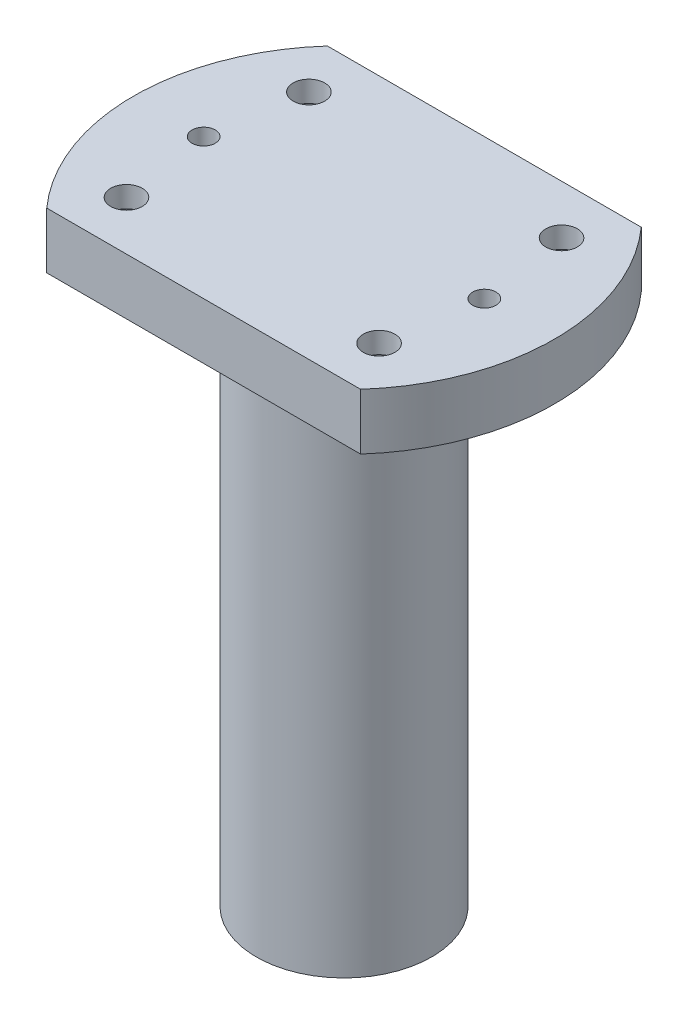
from build123d import *

# Parameters (mm, degrees)
M4_TAPPED_HOLE1_D                       = 3.3
M4_TAPPED_HOLE1_DEPTH                   = 11.5
M4_TAPPED_HOLE1_TIP                     = 0.991420021
CUT_EXTRUDE2_REACH                      = 97
CBORE_FOR_M4_HEX_HEAD_BOLT1_D           = 3
CBORE_FOR_M4_HEX_HEAD_BOLT1_CBORE_D     = 8
CBORE_FOR_M4_HEX_HEAD_BOLT1_CBORE_DEPTH = 3
M4_TAPPED_HOLE4_D                       = 3.3
M4_TAPPED_HOLE4_DEPTH                   = 10.1
M4_TAPPED_HOLE4_TIP                     = 0.991420021
CBORE_FOR_M4_HEX_HEAD_BOLT2_D           = 4.5
CBORE_FOR_M4_HEX_HEAD_BOLT2_DEPTH       = 10.1
CBORE_FOR_M4_HEX_HEAD_BOLT2_CBORE_D     = 8
CBORE_FOR_M4_HEX_HEAD_BOLT2_CBORE_DEPTH = 5
CBORE_FOR_M4_HEX_HEAD_BOLT2_TIP         = 1.351936393


with BuildPart() as part:
    # Sketch1 → Revolve1 (revolve)
    with BuildSketch(Plane.XY, mode=Mode.PRIVATE) as revolve1_sk:
        Polygon((0, 85), (-30, 85), (-30, 77), (-12.5, 77), (-12.5, 0), (0, 0), align=None)
    revolve(revolve1_sk.sketch.rotate(Axis((0, 0, 0), (0, 1, 0)), 270), axis=Axis((0, 0, 0), (0, 1, 0)))

    # M4 Tapped Hole1
    with Locations(Plane(origin=(-8, 0, 0), x_dir=(0, 0, -1), z_dir=(0, -1, 0))):
        with Locations((0, 0), (0, 16)):
            Hole(M4_TAPPED_HOLE1_D / 2, depth=M4_TAPPED_HOLE1_DEPTH)
            with Locations((0, 0, -(M4_TAPPED_HOLE1_DEPTH + M4_TAPPED_HOLE1_TIP / 2))):  # 118° drill point
                Cone(0, M4_TAPPED_HOLE1_D / 2, M4_TAPPED_HOLE1_TIP, mode=Mode.SUBTRACT)

    # Sketch4 → Cut-Extrude2 (cut, up to next)
    with BuildSketch(Plane(origin=(0, 85, 0), x_dir=(1, 0, 0), z_dir=(0, 1, 0)), mode=Mode.PRIVATE) as cut_extrude2_sk1:
        with BuildLine():
            Line((22.360679775, 20), (-22.360679775, 20))
            ThreePointArc((-22.360679775, 20), (0, 30), (22.360679775, 20))
        make_face()
    cut_extrude2_tool1 = extrude(cut_extrude2_sk1.sketch, amount=-CUT_EXTRUDE2_REACH, mode=Mode.PRIVATE) & part.part
    # Sketch4 → Cut-Extrude2 (cut, up to next)
    with BuildSketch(Plane(origin=(0, 85, 0), x_dir=(1, 0, 0), z_dir=(0, 1, 0)), mode=Mode.PRIVATE) as cut_extrude2_sk2:
        with BuildLine():
            Line((22.360679775, -20), (-22.360679775, -20))
            ThreePointArc((-22.360679775, -20), (0, -30), (22.360679775, -20))
        make_face()
    cut_extrude2_tool2 = extrude(cut_extrude2_sk2.sketch, amount=-CUT_EXTRUDE2_REACH, mode=Mode.PRIVATE) & part.part
    add(cut_extrude2_tool1.solids().sort_by_distance((0, 85, -24.063287))[0], mode=Mode.SUBTRACT)
    add(cut_extrude2_tool2.solids().sort_by_distance((0, 85, 24.063287))[0], mode=Mode.SUBTRACT)

    # CBORE for M4 Hex Head Bolt1 (through all)
    with Locations(Plane(origin=(-20, 77, 0), x_dir=(0, 0, -1), z_dir=(0, -1, 0))):
        with Locations((0, 0), (0, 40)):
            CounterBoreHole(CBORE_FOR_M4_HEX_HEAD_BOLT1_D / 2, CBORE_FOR_M4_HEX_HEAD_BOLT1_CBORE_D / 2, CBORE_FOR_M4_HEX_HEAD_BOLT1_CBORE_DEPTH)

    # M4 Tapped Hole4
    with Locations(Plane(origin=(-20, 80, 0), x_dir=(0, 0, -1), z_dir=(0, -1, 0))):
        with Locations((0, 0), (0, 40)):
            Hole(M4_TAPPED_HOLE4_D / 2, depth=M4_TAPPED_HOLE4_DEPTH)
            with Locations((0, 0, -(M4_TAPPED_HOLE4_DEPTH + M4_TAPPED_HOLE4_TIP / 2))):  # 118° drill point
                Cone(0, M4_TAPPED_HOLE4_D / 2, M4_TAPPED_HOLE4_TIP, mode=Mode.SUBTRACT)

    # CBORE for M4 Hex Head Bolt2
    with Locations(Plane(origin=(-18, 77, 13), x_dir=(0, 0, -1), z_dir=(0, -1, 0))):
        with Locations((0, 0), (0, 36), (26, 36), (26, 0)):
            CounterBoreHole(CBORE_FOR_M4_HEX_HEAD_BOLT2_D / 2, CBORE_FOR_M4_HEX_HEAD_BOLT2_CBORE_D / 2, CBORE_FOR_M4_HEX_HEAD_BOLT2_CBORE_DEPTH, depth=CBORE_FOR_M4_HEX_HEAD_BOLT2_DEPTH)
            with Locations((0, 0, -(CBORE_FOR_M4_HEX_HEAD_BOLT2_DEPTH + CBORE_FOR_M4_HEX_HEAD_BOLT2_TIP / 2))):  # 118° drill point
                Cone(0, CBORE_FOR_M4_HEX_HEAD_BOLT2_D / 2, CBORE_FOR_M4_HEX_HEAD_BOLT2_TIP, mode=Mode.SUBTRACT)


solid = part.part
